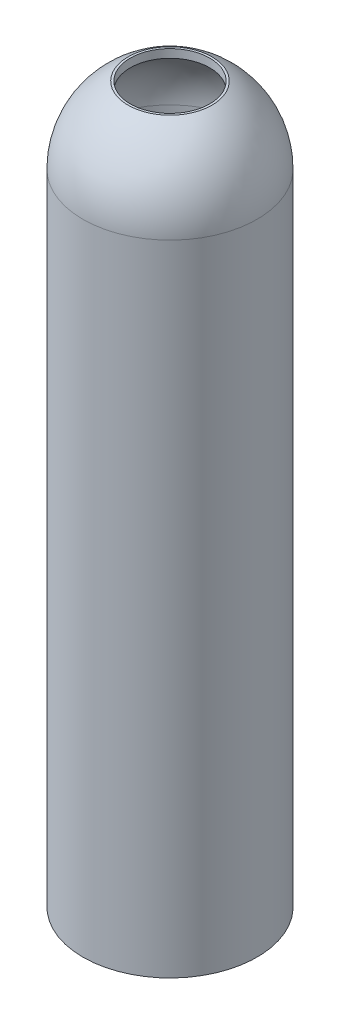
SolidWorks part; units mm, degrees
material "铁"
ref_plane "Front Plane" through (0, 0, 0) normal (0, 0, 1) x (1, 0, 0)
ref_plane "Top Plane" through (0, 0, 0) normal (0, 1, 0) x (1, 0, 0)
ref_plane "Right Plane" through (0, 0, 0) normal (1, 0, 0) x (0, 0, -1)
sketch "Sketch1" plane through (0, 0, 0) normal (0, 0, 1) x (1, 0, 0)
  line L0 (0, 0) -> (0, 25.3635) construction
  line L1 (-2.18, 0) -> (-2.18, 16)
  line L2 (-1.05, 17.9105) -> (-0.9946, 17.9105)
  line L3 (-1.97, 0) -> (-1.97, 16)
  line L5 (-2.18, 0) -> (-1.97, 0)
  line L7 (-0.9946, 17.7005) -> (-0.9946, 17.9105)
  line L9 (0, 17.9105) -> (-1.05, 17.9105) construction
  line L10 (0, 17.7005) -> (-0.9946, 17.7005) construction
  arc A0 (-2.18, 16) -> (-1.05, 17.9105) centre (0, 16) cw
  arc A1 (-1.97, 16) -> (-0.9946, 17.7005) centre (0, 16) cw
  arc A2 (-2.18, 16) -> (-1.05, 17.9105) centre (0, 16) cw construction
  dimension "D2" = 2.18
  dimension "D1" = 4.36
  dimension "D3" = 16
  dimension "D4" = 1.9893
  dimension "D5" = 0.21
revolve "Revolve1" add sketch "Sketch1" angle 360 about L0
